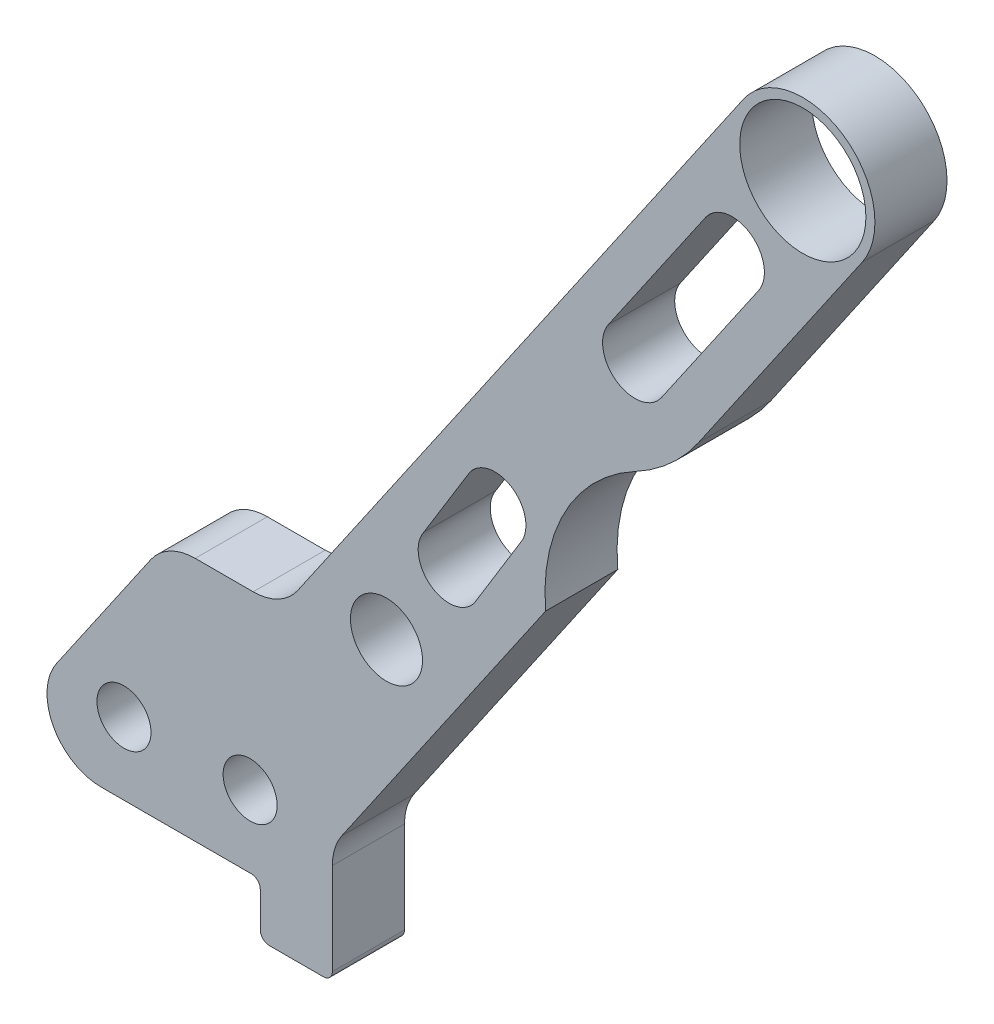
from build123d import *

# Parameters (mm, degrees)
SKETCH1_R           = 15
SKETCH1_R_2         = 20
SKETCH1_R_3         = 35
BOSS_EXTRUDE1_DEPTH = 40


with BuildPart() as part:
    # Sketch1 → Boss-Extrude1 (new body)
    with BuildSketch(Plane.XY):
        with BuildLine():
            Line((136298.479378134, -173227.631246443), (136051.215190424, -173587.288246748))
            ThreePointArc((136051.215190424, -173587.288246748), (136040.460393586, -173596.843050045), (136026.493932699, -173600.292382063))
            Line((136026.493932699, -173600.292382063), (135994.358099543, -173600.292382063))
            ThreePointArc((135994.358099543, -173600.292382063), (135980.391638657, -173603.741714079), (135969.636841818, -173613.296517373))
            Line((135969.636841818, -173613.296517373), (135917.386841817, -173689.296517375))
            ThreePointArc((135917.386841817, -173689.296517375), (135915.557431558, -173720.258842949), (135942.10809954, -173736.292382064))
            Line((135942.10809954, -173736.292382064), (136025.44105537, -173736.292382064))
            ThreePointArc((136025.44105537, -173736.292382064), (136028.976589274, -173737.756848164), (136030.44105537, -173741.29238207))
            Line((136030.44105537, -173741.29238207), (136030.44105537, -173760.79238207))
            ThreePointArc((136030.44105537, -173760.79238207), (136031.905521462, -173764.327915975), (136035.441055367, -173765.79238207))
            Line((136035.441055367, -173765.79238207), (136065.44105537, -173765.79238207))
            ThreePointArc((136065.44105537, -173765.79238207), (136068.976589275, -173764.327915968), (136070.441055364, -173760.792382057))
            Line((136070.441055364, -173760.792382057), (136070.441055364, -173709.851867037))
            ThreePointArc((136070.441055364, -173709.851867037), (136071.791118787, -173700.953488864), (136075.71979764, -173692.856002351))
            Line((136075.71979764, -173692.856002351), (136188.781239342, -173528.402996239))
            ThreePointArc((136188.781239342, -173528.402996239), (136199.652035077, -173475.031986515), (136238.252029422, -173436.60440117))
            ThreePointArc((136238.252029422, -173436.60440117), (136257.830557919, -173422.935627875), (136273.610475811, -173405.01501592))
            Line((136273.610475811, -173405.01501592), (136364.402732332, -173272.953551889))
            ThreePointArc((136364.402732332, -173272.953551889), (136354.102207956, -173217.330722066), (136298.479378134, -173227.631246443))
        make_face()
        with Locations((136024.816066991, -173696.292382064)):
            Circle(SKETCH1_R, mode=Mode.SUBTRACT)
        with Locations((135954.816066991, -173696.292382064)):
            Circle(SKETCH1_R, mode=Mode.SUBTRACT)
        with Locations((136100.44105537, -173586.292398967)):
            Circle(SKETCH1_R_2, mode=Mode.SUBTRACT)
        with Locations((136331.44105537, -173250.292398967)):
            Circle(SKETCH1_R_3, mode=Mode.SUBTRACT)
        with BuildLine():
            Line((136121.226562597, -173524.21041858), (136146.693938197, -173482.735767799))
            ThreePointArc((136146.693938197, -173482.735767799), (136169.679901616, -173478.163942115), (136175.848114544, -173500.773879171))
            Line((136175.848114544, -173500.773879171), (136150.47388525, -173542.2345113))
            ThreePointArc((136150.47388525, -173542.2345113), (136126.210129016, -173548.865247662), (136121.226562597, -173524.21041858))
        make_face(mode=Mode.SUBTRACT)
        with BuildLine():
            Line((136223.494638872, -173373.447446962), (136277.473587055, -173294.932613241))
            ThreePointArc((136277.473587055, -173294.932613241), (136302.376683609, -173290.320928694), (136306.988368156, -173315.224025248))
            Line((136306.988368156, -173315.224025248), (136253.009419973, -173393.738858969))
            ThreePointArc((136253.009419973, -173393.738858969), (136228.106323419, -173398.350543516), (136223.494638872, -173373.447446962))
        make_face(mode=Mode.SUBTRACT)
    extrude(amount=BOSS_EXTRUDE1_DEPTH)


solid = part.part
